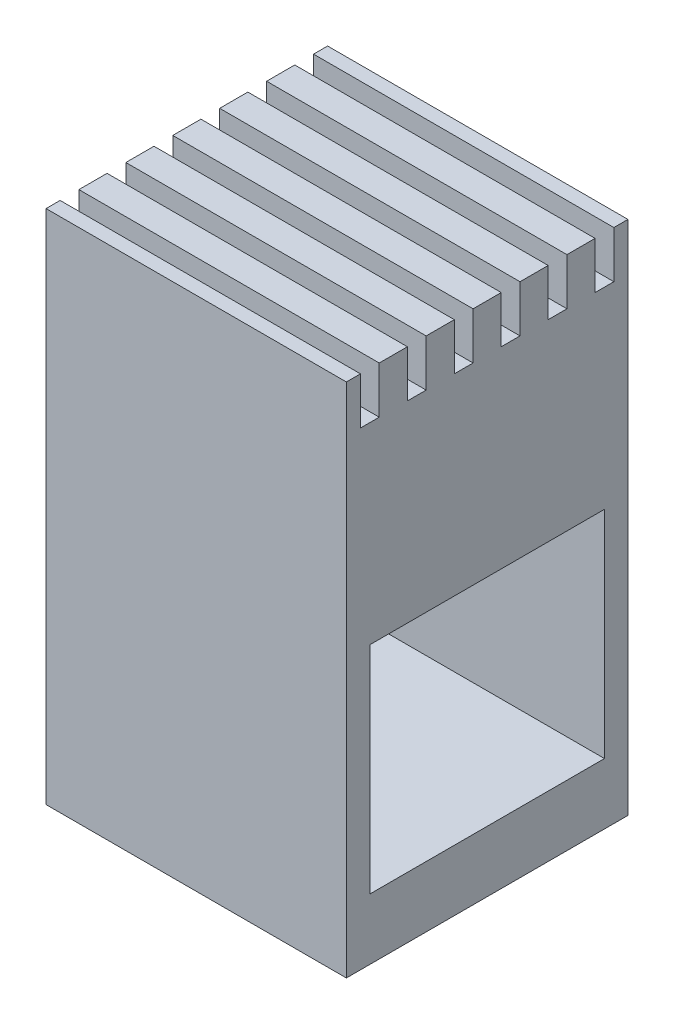
SolidWorks part; units mm, degrees
ref_plane "前视基准面" through (0, 0, 0) normal (0, 0, 1) x (1, 0, 0)
ref_plane "上视基准面" through (0, 0, 0) normal (0, 1, 0) x (1, 0, 0)
ref_plane "右视基准面" through (0, 0, 0) normal (1, 0, 0) x (0, 0, -1)
sketch "草图1" plane through (0, 0, 0) normal (0, 1, 0) x (1, 0, 0)
  line L1 (-16, 15) -> (16, 15)
  line L2 (-16, 15) -> (-16, -15)
  line L3 (-16, -15) -> (16, -15)
  line L4 (16, 15) -> (16, -15)
  line L5 (-16, 15) -> (16, -15) construction
  line L6 (-16, -15) -> (16, 15) construction
  point P0 (0, 0)
  dimension "D1" = 32
  dimension "D2" = 30
extrude "凸台-拉伸1" add sketch "草图1" along normal blind 55
hole_wizard "M3 螺纹孔1" positions "草图3" profile "草图4" tap size "M3" standard "GB"
sketch "草图3" plane through (0, 0, 0) normal (0, -1, 0) x (-1, 0, 0)
  line L1 (-16, -15) -> (-16, 15) construction
  point P24 (9, 7.5)
  point P26 (9, -7.5)
  dimension "D1" = 25
  dimension "D2" = 15
  dimension "D3" = 7.5
sketch "草图4" plane through (-9, 0, -7.5) normal (1, 0, 0) x (0, 0, -1)
  line L0 (0, 0) -> (0, 8.2511)
  line L1 (0, 8.2511) -> (1.25, 7.5)
  line L2 (1.25, 7.5) -> (1.25, 0)
  line L5 (1.25, 0) -> (0, 0)
  line L10 (0, 8.2511) -> (-1.25, 7.5) construction
  line L11 (0, -6.35) -> (0, 107.95) construction
  dimension "螺纹孔钻头直径" = 2.5
  dimension "螺纹孔钻头深度" = 7.5
  dimension "导头角度" = 118
cosmetic thread "孔螺蚊线3" parameters "D1"=6, "D2"=3
cosmetic thread "孔螺蚊线4" parameters "D1"=6, "D2"=3
sketch "草图5" plane through (16, 0, 0) normal (1, 0, 0) x (0, 0, -1)
  line L0 (-15, 0) -> (15, 0) construction
  line L1 (-12.5, 6.5) -> (12.5, 6.5)
  line L2 (-12.5, 6.5) -> (-12.5, 29.5)
  line L3 (-12.5, 29.5) -> (12.5, 29.5)
  line L4 (12.5, 6.5) -> (12.5, 29.5)
  dimension "D1" = 23
  dimension "D2" = 25
  dimension "D3" = 12.5
  dimension "8" = 6.5
extrude "切除-拉伸2" cut sketch "草图5" against normal blind 60
sketch "草图6" plane through (16, 0, 0) normal (1, 0, 0) x (0, 0, -1)
  line L0 (-15, 55) -> (15, 55) construction
  line L1 (-13.5, 55) -> (-11.5, 55)
  line L2 (-13.5, 55) -> (-13.5, 50)
  line L3 (-13.5, 50) -> (-11.5, 50)
  line L4 (-11.5, 55) -> (-11.5, 50)
  line L5 (-15, 55) -> (-15, 0) construction
  dimension "D1" = 2
  dimension "D2" = 5
  dimension "D3" = 1.5
extrude "切除-拉伸3" cut sketch "草图6" against normal through all
pattern_linear "阵列(线性)1" count 6 spacing 5 along (0, 0, -1) of "切除-拉伸3"
